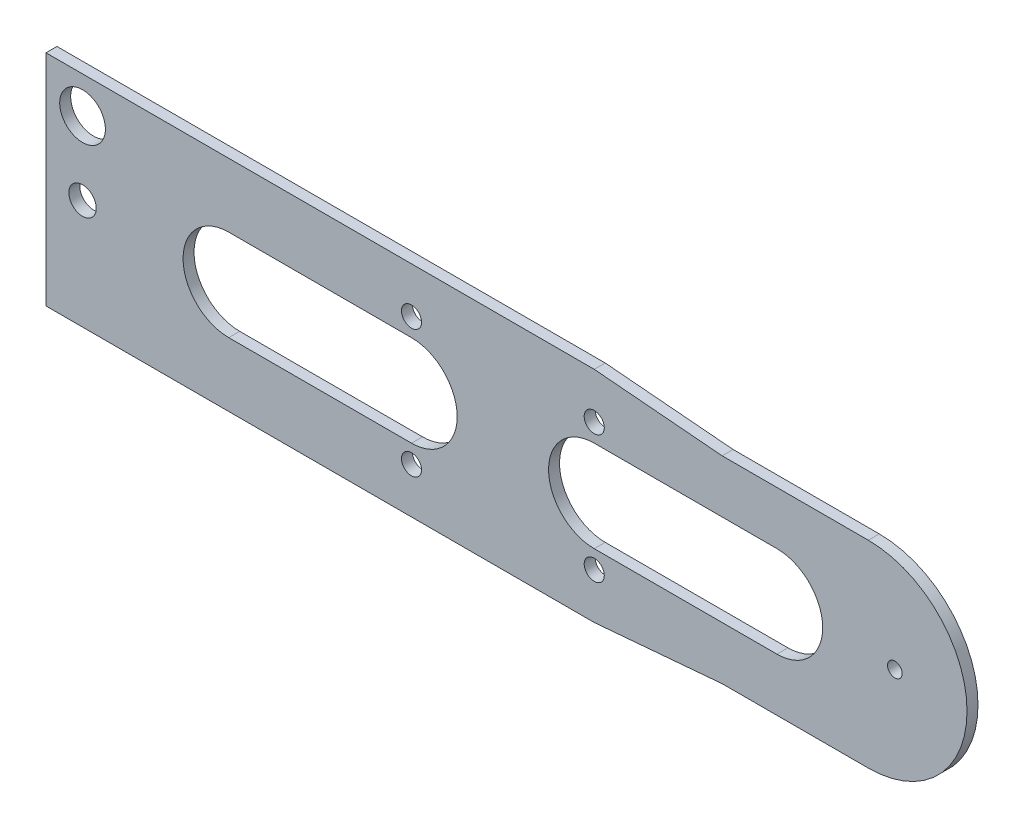
from build123d import *

# Parameters (mm, degrees)
SKETCH_1_R                   = 12.5
SKETCH_1_R_2                 = 7.5
EXTRUDE_1_DEPTH              = 6
HOLE_WIZARD_M6_1_D           = 7
HOLE_WIZARD_M6_1_CBORE_D     = 11
HOLE_WIZARD_M6_1_CBORE_DEPTH = 6.8
SKETCH_7_R                   = 4
CUT_EXTRUDE_1_DEPTH          = 10


with BuildPart() as part:
    # 草图1 → 凸台-拉伸1 (new body)
    with BuildSketch(Plane.XY):
        with BuildLine():
            Line((-255, 0), (45, 0))
            Line((45, 0), (115, 6))
            Line((115, 6), (195, 6))
            ThreePointArc((195, 6), (249, 60), (195, 114))
            Line((195, 114), (115, 114))
            Line((115, 114), (45, 120))
            Line((45, 120), (-235, 120))
            Line((-235, 120), (-255, 120))
            Line((-255, 120), (-255, 0))
        make_face()
        with Locations((-235, 100)):
            Circle(SKETCH_1_R, mode=Mode.SUBTRACT)
        with Locations((-235, 60)):
            Circle(SKETCH_1_R_2, mode=Mode.SUBTRACT)
        with BuildLine():
            Line((-155, 85), (-55, 85))
            ThreePointArc((-55, 85), (-30, 60), (-55, 35))
            Line((-55, 35), (-155, 35))
            ThreePointArc((-155, 35), (-180, 60), (-155, 85))
        make_face(mode=Mode.SUBTRACT)
        with BuildLine():
            Line((45, 85), (145, 85))
            ThreePointArc((145, 85), (170, 60), (145, 35))
            Line((145, 35), (45, 35))
            ThreePointArc((45, 35), (20, 60), (45, 85))
        make_face(mode=Mode.SUBTRACT)
    extrude(amount=EXTRUDE_1_DEPTH)

    # M6 六角圆柱头螺钉的柱形沉头孔1 (through all)
    with Locations(Plane.XY.offset(6)):
        with Locations((-55, 95), (-55, 25), (45, 95), (45, 25)):
            CounterBoreHole(HOLE_WIZARD_M6_1_D / 2, HOLE_WIZARD_M6_1_CBORE_D / 2, HOLE_WIZARD_M6_1_CBORE_DEPTH)

    # 草图7 → 切除-拉伸1 (cut)
    with BuildSketch(Plane(origin=(0, 0, 0), x_dir=(-1, 0, 0), z_dir=(0, 0, -1))):
        with Locations((-209.5, 60)):
            Circle(SKETCH_7_R)
    extrude(amount=-CUT_EXTRUDE_1_DEPTH, mode=Mode.SUBTRACT)


solid = part.part
